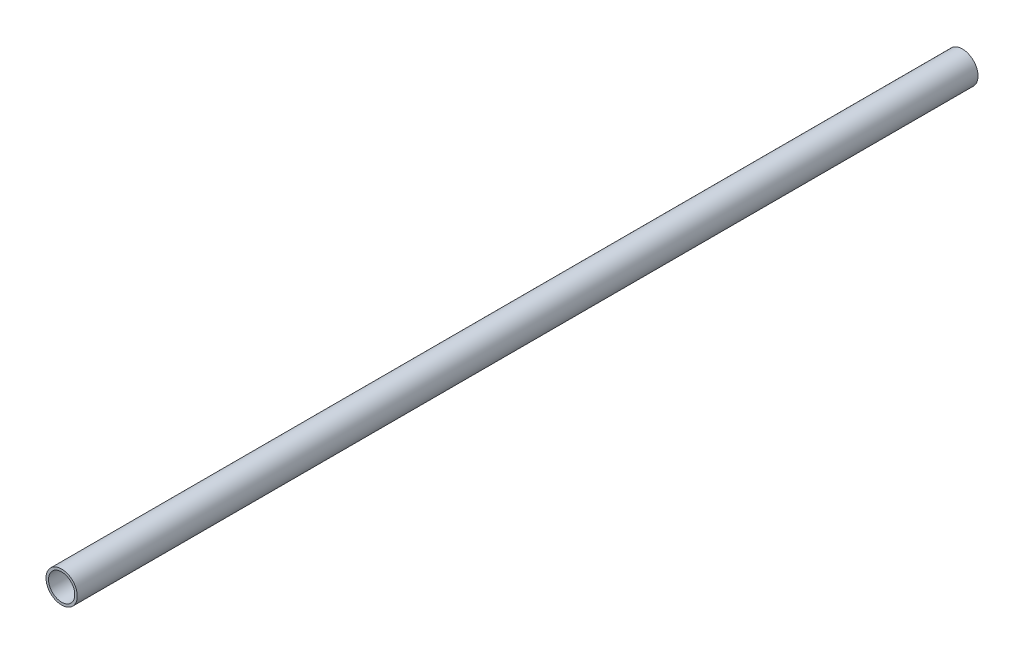
SolidWorks part; units mm, degrees
ref_plane "前视基准面" through (0, 0, 0) normal (0, 0, 1) x (1, 0, 0)
ref_plane "上视基准面" through (0, 0, 0) normal (0, 1, 0) x (1, 0, 0)
ref_plane "右视基准面" through (0, 0, 0) normal (1, 0, 0) x (0, 0, -1)
sketch "草图1" plane through (0, 0, 0) normal (0, 0, 1) x (1, 0, 0)
  circle A0 centre (0, 0) radius 12.5
  circle A1 centre (0, 0) radius 10.5
  dimension "D1" = 25
  dimension "D2" = 2
extrude "凸台-拉伸1" add sketch "草图1" along normal mid plane 720
